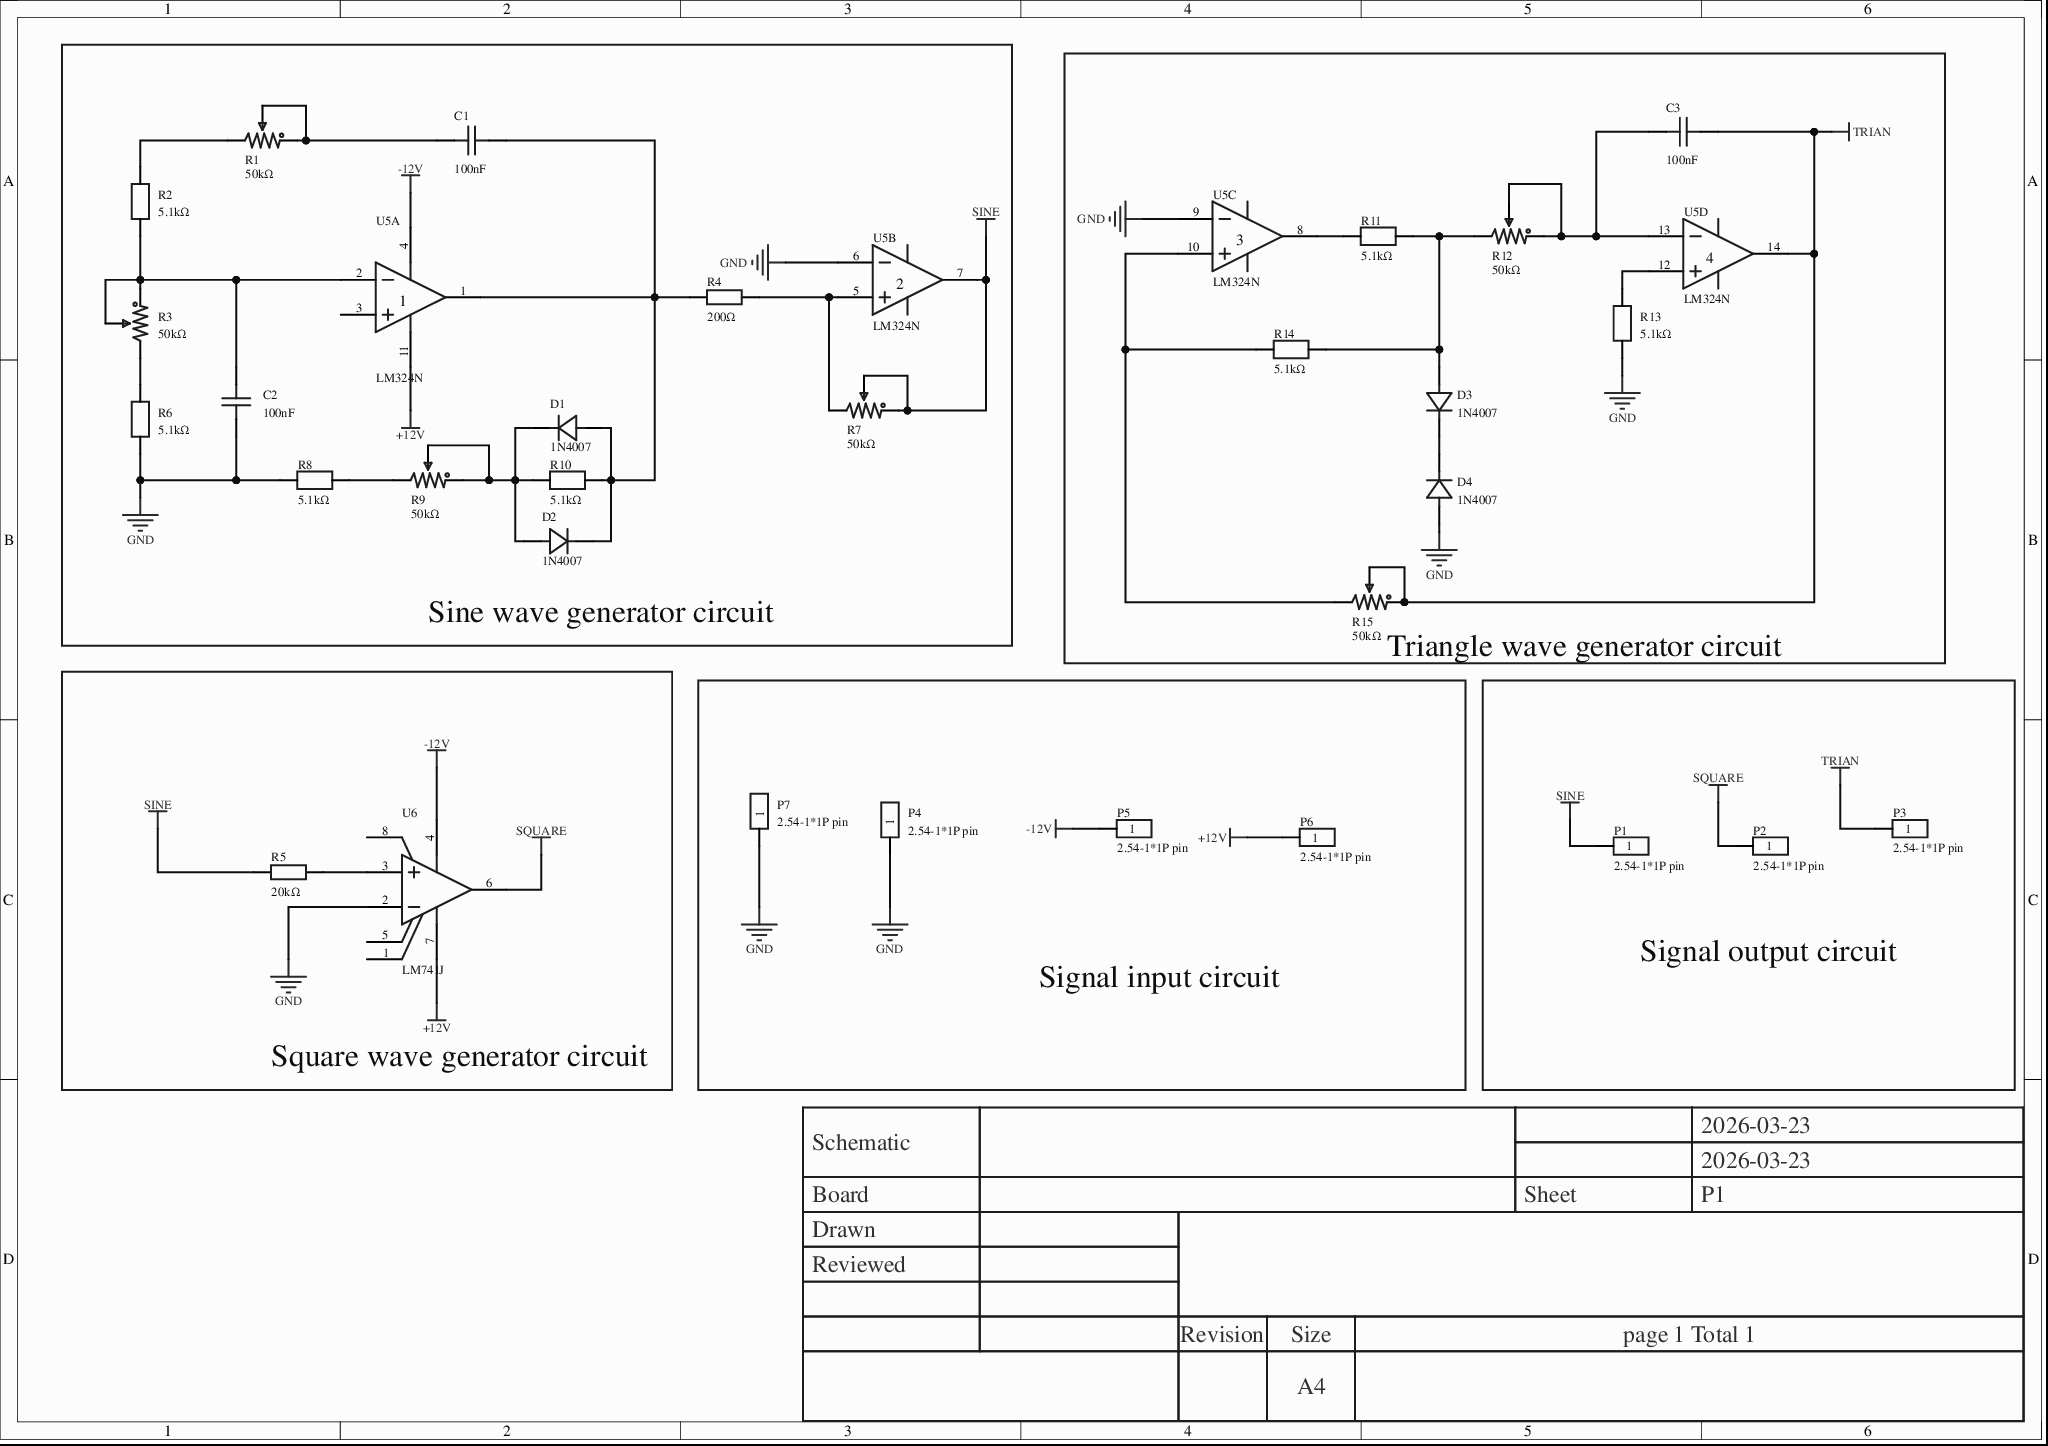
[diagram p0: MISC51008-3.schdoc]
# Altium project MISC51008-2.PrjPcb
1 sheet, 31 parts. Net scope: global (net labels, ports and power ports of the same name join across sheets).
Board file: MISC51008.pcbdoc

## Sheet MISC51008-3.schdoc
size 297 x 209 mm; Version: V1.0; @Project Name: MISC51008; @Update Date: 2026-05-11; @Create Date: 2026-05-11; @Board Name: MISC51008; @Create Time: 16:13:02; @Page Count: 1; @Page No: 1; @Schematic Name: MISC51008; @Update Time: 16:13:02; Size: A4

### Parts
C1  100nF  [C0603]
C2  100nF  [C0603]
C3  100nF  [C0603]
D1  1N4007  [SMA_L4.3-W2.5-LS5.0-RD]
D2  1N4007  [SMA_L4.3-W2.5-LS5.0-RD-1]
D3  1N4007  [SMA_L4.3-W2.5-LS5.0-RD]
D4  1N4007  [SMA_L4.3-W2.5-LS5.0-RD]
P1  2.54-1*1P pin  [HDR-TH_1P-P2.54-V-M]
P2  2.54-1*1P pin  [HDR-TH_1P-P2.54-V-M]
P3  2.54-1*1P pin  [HDR-TH_1P-P2.54-V-M]
P4  2.54-1*1P pin  [HDR-TH_1P-P2.54-V-M]
P5  2.54-1*1P pin  [HDR-TH_1P-P2.54-V-M]
P6  2.54-1*1P pin  [HDR-TH_1P-P2.54-V-M]
P7  2.54-1*1P pin  [HDR-TH_1P-P2.54-V-M]
R1  50kΩ  [RES-ADJ-TH_3P-L9.5-W4.85-P2.50-BL-BS]
R2  5.1kΩ  [R0603]
R3  50kΩ  [RES-ADJ-TH_3P-L9.5-W4.85-P2.50-BL-BS]
R4  200Ω  [R0603]
R5  20kΩ  [R0603]
R6  5.1kΩ  [R0603]
R7  50kΩ  [RES-ADJ-TH_3P-L9.5-W4.85-P2.50-BL-BS]
R8  5.1kΩ  [R0603]
R9  50kΩ  [RES-ADJ-TH_3P-L9.5-W4.85-P2.50-BL-BS]
R10  5.1kΩ  [R0603]
R11  5.1kΩ  [R0603]
R12  50kΩ  [RES-ADJ-TH_3P-L9.5-W4.85-P2.50-BL-BS]
R13  5.1kΩ  [R0603]
R14  5.1kΩ  [R0603]
R15  50kΩ  [RES-ADJ-TH_3P-L9.5-W4.85-P2.50-BL-BS]
U5  LM324N  [DIP-14_L19.4-W6.4-P2.54-LS7.6-BL]  (parts A,B,C,D of 4)
U6  LM741J  [CDIP-8_L10.3-W6.7-P2.54-LS7.6-BL]

### Blocks framed on the sheet
Sine wave generator circuit: C1 C2 D1 D2 R1-R4 R6-R10 U5
Triangle wave generator circuit: C3 D3 D4 R11-R15 U5
Square wave generator circuit: R5 U6
Signal output circuit: P1-P3

### Nets
+12V: P6.1 U5.11(GND) U6.7(V+)
-12V: P5.1 U5.4(VCC) U6.4(V-)
GND: C2.1 D4.2(A) P4.1 P7.1 R6.1 R8.1 R13.1 U5.6(IN2-) U5.9(IN3-) U6.2(IN-)
SINE: P1.1 R5.1 R7.1 R7.2 U5.7(OUT2)
SQUARE: P2.1 U6.6(OUT)
TRIAN: C3.2 P3.1 R15.1 R15.2 U5.14(OUT4)
NetC1_1: C1.1 R1.1 R1.2
NetC1_2: C1.2 D1.2(A) D2.1(K) R4.1 R10.2 U5.1(OUT1)
NetC2_2: C2.2 R2.1 R3.1 R3.2 U5.2(IN1-)
NetC3_1: C3.1 R12.1 R12.2 U5.13(IN4-)
NetD1_1: D1.1(K) D2.2(A) R9.1 R9.2 R10.1
NetD3_1: D3.1(K) D4.1(K)
NetD3_2: D3.2(A) R11.2 R12.3 R14.2
NetR1_3: R1.3 R2.2
NetR3_3: R3.3 R6.2
NetR4_2: R4.2 R7.3 U5.5(IN2+)
NetR5_2: R5.2 U6.3(IN+)
NetR8_2: R8.2 R9.3
NetR11_1: R11.1 U5.8(OUT3)
NetR13_2: R13.2 U5.12(IN4+)
NetR14_1: R14.1 R15.3 U5.10(IN3+)

Not connected (* = marked no-connect by the designer): U5 3(IN1+); U6 1(OFFSET_NULL)* 5(OFFSET_NULL)* 8(NC)*

### Notes on the sheet
- Signal input circuit
- 2026-03-23
- Schematic
- Board
- Sheet
- P1
- Drawn
- Reviewed
- Revision
- Size
- A4
- page 1 Total 1

### Library data of the parts
C1-C3 = CGA0603X7R104K500JT: Manufacturer: HRE(芯声); AddInBom: yes; Tolerance: ±10%; Voltage Rating: 50V; Temperature Coefficient: X7R; ModelId: ac125912035d415993ca9572d50418b10819f05c4eef4c71ace90d822a990e87; ModelName: C0603_L1.6-W0.8-H0.8; ModelTransform: 62.992,31.496,0,0,0,0,0,0,0; Device: CGA0603X7R104K500JT; Symbol: CGA0603X7R104K500JT; FootprintName: C0603; LCSC Part Name: 100nF ±10% 50V; SupplierPart: C6119867; ManufacturerPart: CGA0603X7R104K500JT; Supplier Footprint: 0603; JLCPCB Part Class: Extended Part; Datasheet: https://example.com/datasheet/CGA0603X7R104K500JT/7062573.html; Supplier: LCSC; ConvertToPcb: yes; Value: 100nF
D1 D2 = 1N4007_C2985028: Manufacturer: GOODWORK(固得沃克); AddInBom: yes; Diode Configuration: Discrete; Voltage - Forward(Vf@If): 1V@1A; Voltage - DC Reverse(Vr): 1kV; Current - Rectified: 1A; Reverse Leakage Current (Ir): 5uA@1kV; Non-Repetitive Peak Forward Surge Current: 30A; Operating Junction Temperature Range: -65℃~+150℃; ModelId: 6de1e9b71a0d4751b4e9df530304c1a30819f05c4eef4c71ace90d822a990e87; ModelName: DO-41_D2.4-L4.7-P8.70; ModelTransform: 374.015,94.428,0,0,0,0,0,0,-137.795; Device: 1N4007_C2985028; Symbol: 1N4007_C2985028; LCSC Part Name: 电压:1kV 电流:1A; SupplierPart: C2985028; ManufacturerPart: 1N4007; Supplier Footprint: DO-41; JLCPCB Part Class: Extended Part; Datasheet: https://example.com/datasheet/1N4007/3428711.html; Supplier: LCSC; ConvertToPcb: yes
  D1: FootprintName: SMA_L4.3-W2.5-LS5.0-RD
  D2: FootprintName: SMA_L4.3-W2.5-LS5.0-RD-1
D3 D4 = 1N4007_C727081: Manufacturer: TWGMC(迪嘉); AddInBom: yes; Diode Configuration: Discrete; Voltage - Forward(Vf@If): 1.1V@1A; Voltage - DC Reverse(Vr): 1kV; Current - Rectified: 1A; Reverse Leakage Current (Ir): 5uA; ModelId: 5b53cc1b87a148cc9fa13125be89f9480819f05c4eef4c71ace90d822a990e87; ModelTransform: 194.8815,98.425,0,0,0,0,0,0,0; Device: 1N4007_C727081; Symbol: 1N4007_C727081; FootprintName: SMA_L4.3-W2.5-LS5.0-RD; LCSC Part Name: 1N4007; SupplierPart: C727081; ManufacturerPart: 1N4007; Supplier Footprint: SMA(DO-214AC); JLCPCB Part Class: Extended Part; Datasheet: https://example.com/datasheet/1N4007/774186.html; Supplier: LCSC; ConvertToPcb: yes; ModelName: SMA_L4.3-W2.5-LS5.0-RD
P1-P7 = 2.54-1*1P针: Manufacturer: BOOMELE(博穆精密); Symbol: Header-Male-2.54_1x1; AddInBom: yes; Pin Structure: 1x1P; Circluar Pins/Square Pins: Square pin; Current Rating: 3A; ModelId: efa57846279b44bfa0a28253a2c74e330819f05c4eef4c71ace90d822a990e87; ModelName: HDR2.54-M-LI-1X1P; ModelTransform: 100,100,0,0,0,0,0,0,-118.11; Device: 2.54-1*1P pin; FootprintName: HDR-TH_1P-P2.54-V-M; LCSC Part Name: 1x1P 方针 直插; SupplierPart: C81276; ManufacturerPart: 2.54-1*1P针; Supplier Footprint: 插件,P=2.54mm; JLCPCB Part Class: Extended Part; Datasheet: https://example.com/datasheet/2.54-1*1P%25E9%2592%2588/82426.html; Supplier: LCSC; ConvertToPcb: yes; Pitch: -; Row Spacing: -; Mounting Type: Through-hole; Number of Rows: Single row; Number of Pins: 1P; Voltage Rating (Max): -; Length of Mating Pin: 6mm; Insulation Height: 2.5mm; Length of End Connection Pin: 3mm; Contact Material: Brass; Contact Plating: Gold; Operating Temperature: -55℃~+105℃; Color: Black
R1 R3 R7 R9 R12 R15 = 3296W-1-503_C48997928: Manufacturer: JIERR(捷而瑞); AddInBom: yes; Tolerance: ±10%; Power(Watts): 500mW; Temperature Coefficient: ±250ppm/℃; Number of Turns: 28; ModelId: b182808559bb43bda9e7de64b64134cb0819f05c4eef4c71ace90d822a990e87; ModelName: 3296W; ModelTransform: 374.015,188.976,0,90,0,0,0,0,-137.795; Device: 3296W-1-503_C48997928; Symbol: 3296W-1-503_C48997928; FootprintName: RES-ADJ-TH_3P-L9.5-W4.85-P2.50-BL-BS; LCSC Part Name: 3296W-1-503; SupplierPart: C48997928; ManufacturerPart: 3296W-1-503; Supplier Footprint: 插件-3P,9.5x4.9mm; JLCPCB Part Class: Extended Part; Datasheet: https://example.com/datasheet/3296W-1-503/51342064.html; Supplier: LCSC; ConvertToPcb: yes; Value: 50kΩ
R2 R6 R8 R10 R11 R13 R14 = FRC0603F5101TS: Manufacturer: FOJAN(富捷); AddInBom: yes; Tolerance: ±1%; Power(Watts): 100mW; Voltage-Supply(Max): 75V; Temperature Coefficient: ±100ppm/℃; ModelId: fc143cca1e79419f9cd78b61e9279f080819f05c4eef4c71ace90d822a990e87; ModelTransform: 31.8897,63.7794,0,90,0,0,0,0,0; Device: FRC0603F5101TS; Symbol: FRC0603F5101TS; FootprintName: R0603; LCSC Part Name: 5.1kΩ ±1% 100mW 厚膜电阻; SupplierPart: C2907044; ManufacturerPart: FRC0603F5101TS; Supplier Footprint: 0603; JLCPCB Part Class: Extended Part; Supplier: LCSC; ConvertToPcb: yes; Type: Thick film resistor; Value: 5.1kΩ; Operating Temperature: -55℃~+155℃; ModelName: R0603
R4 = 0603WAF2000T5E: Manufacturer: UNI-ROYAL(厚声); AddInBom: yes; Tolerance: ±1%; Power(Watts): 100mW; Voltage-Supply(Max): 75V; Temperature Coefficient: ±100ppm/℃; ModelId: fc143cca1e79419f9cd78b61e9279f080819f05c4eef4c71ace90d822a990e87; ModelTransform: 31.8897,63.7794,0,90,0,0,0,0,0; Device: 0603WAF2000T5E; Symbol: 0603WAF2000T5E; FootprintName: R0603; LCSC Part Name: 200Ω ±1% 100mW 厚膜电阻; SupplierPart: C8218; ManufacturerPart: 0603WAF2000T5E; Supplier Footprint: 0603; JLCPCB Part Class: Basic Part; Datasheet: https://example.com/datasheet/0603WAF2000T5E/8708.html; Supplier: LCSC; ConvertToPcb: yes; Type: Thick film resistor; Value: 200Ω; Operating Temperature: -55℃~+155℃; ModelName: R0603
R5 = 0603WAF2002T5E: Manufacturer: UNI-ROYAL(厚声); AddInBom: yes; Tolerance: ±1%; Power(Watts): 100mW; Voltage-Supply(Max): 75V; Temperature Coefficient: ±100ppm/℃; ModelId: fc143cca1e79419f9cd78b61e9279f080819f05c4eef4c71ace90d822a990e87; ModelTransform: 31.8897,63.7794,0,90,0,0,0,0,0; Device: 0603WAF2002T5E; Symbol: 0603WAF2002T5E; FootprintName: R0603; LCSC Part Name: 20kΩ ±1% 100mW 厚膜电阻; SupplierPart: C4184; ManufacturerPart: 0603WAF2002T5E; Supplier Footprint: 0603; JLCPCB Part Class: Basic Part; Datasheet: https://example.com/datasheet/0603WAF2002T5E/4591.html; Supplier: LCSC; ConvertToPcb: yes; Type: Thick film resistor; Value: 20kΩ; Operating Temperature: -55℃~+155℃; ModelName: R0603
U5 = LM324N_C725320: Amplifier count: quad; rail-to-rail: -; gain bandwidth product (GBP): -; input offset voltage (Vos): 9mV; slew rate (SR): -; input bias current (Ib): 250nA;; Manufacturer: HGSEMI(华冠); Relevance: []; 3D Model: 4bcd59468cdc49288dfe5d29f23580610819f05c4eef4c71ace90d822a990e87; 3D Model Transform: 775.19522,311.8104,0,0,0,0,0,-0.02,-118.11; Maximum Power Supply Range (Vdd-Vss): 30V; Input Offset Voltage Drift(Vos TC): 7uV/℃; Input Offset Current(Ios): 50nA; Common Mode Rejection Ratio(CMRR): 80dB; Quiescent Current: 600uA; Output Current: 35mA; Single supply: 1.5V~30V; Dual Supply: -16V~-1.5V; 1.5V~16V; AddInBom: yes; ModelName: DIP-14_L19.4-W6.4-H5.3-P2.54-LS7.6-BL; Device: LM324N_C725320; Symbol: LM324N_C725320; LCSC Part Name: 四路运算放大器; Supplier Part: C725320; Manufacturer Part: LM324N; Supplier Footprint: DIP-14; JLCPCB Part Class: Extended Part; Datasheet: https://example.com/datasheet/LM324N/771554.html; Supplier: LCSC; Number of Channels: Quad; Rail to Rail: -; Gain Bandwidth Product: -; Vos - Input Offset Voltage: 9mV; Slew Rate: -; Ib - Input Bias Current: 250nA; Noise density(eN): -; Input offset current drift(Ios TC): -; Operating Temperature: -40℃~+85℃; FootprintName: DIP-14_L19.4-W6.4-P2.54-LS7.6-BL; ConvertToPcb: yes
U6 = LM741J: Manufacturer: TI(德州仪器); AddInBom: yes; Number of Circuits: Single channel; Gain Bandwidth Product(GBP): 1.5MHz; Slew Rate(SR): 0.5V/us; Current - Input Bias(Ib): 80nA; Output Current: 25mA; ModelId: 9d4740fecfc74f45b7ca88cf9bdf95ec0819f05c4eef4c71ace90d822a990e87; ModelName: CDIP-8_L10.3-W6.7-H4.5-P2.54-LS7.6-BL; ModelTransform: 364.173,311.8104,0,0,0,0,0,0,-118.11; Device: LM741J; Symbol: LM741J; FootprintName: CDIP-8_L10.3-W6.7-P2.54-LS7.6-BL; LCSC Part Name: LM741J; SupplierPart: C1346289; ManufacturerPart: LM741J; Supplier Footprint: CERDIP-8; JLCPCB Part Class: Extended Part; Supplier: LCSC; ConvertToPcb: yes; Operating Temperature: -55℃~+125℃